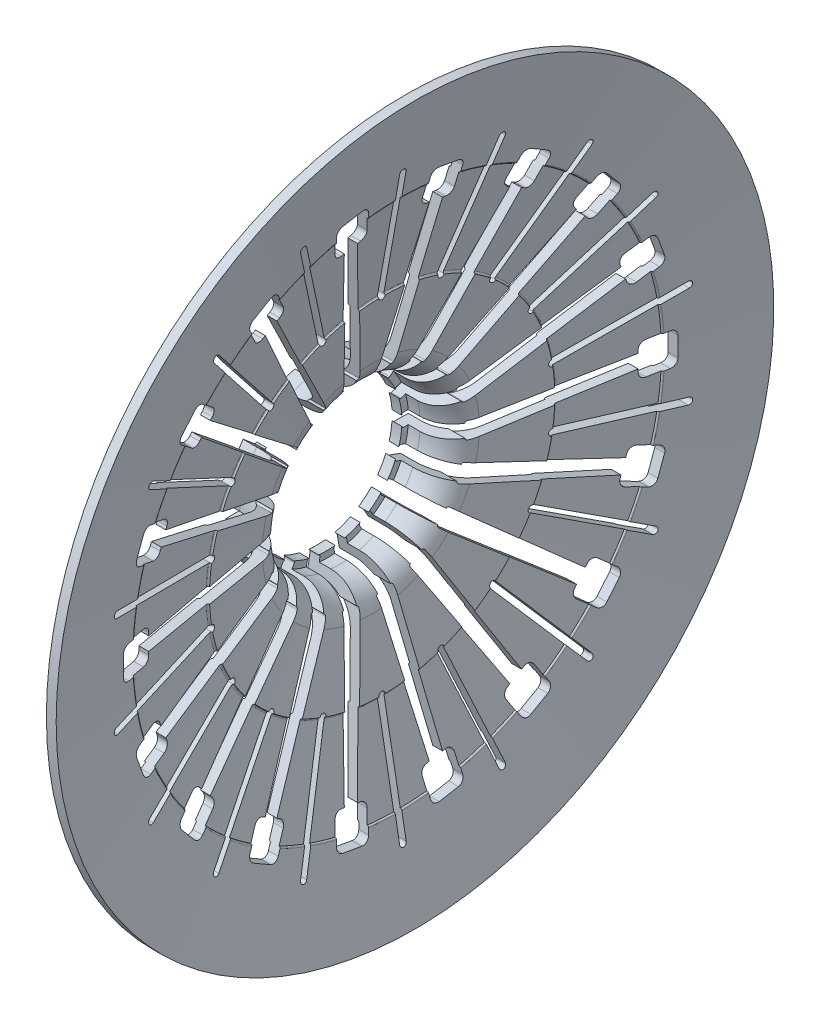
from build123d import *

# Parameters (mm, degrees)
CUT_EXTRUDE3_DEPTH = 1469.5
CUT_EXTRUDE4_DEPTH = 538.860152276
SKETCH10_R         = 23
CUT_EXTRUDE5_DEPTH = 538.860152276
CIRPATTERN3_COUNT  = 18


with BuildPart() as part:
    # Sketch2 → Revolve1 (revolve)
    with BuildSketch(Plane.XY, mode=Mode.PRIVATE) as revolve1_sk:
        with BuildLine():
            Line((1418.670249885, 525.636322255), (1415.670249885, 525.636322255))
            Line((1415.670249885, 525.636322255), (1410.645316665, 497.138509845))
            ThreePointArc((1410.645316665, 497.138509845), (1410.473894028, 496.843629316), (1410.153261537, 496.727289069))
            Line((1410.153261537, 496.727289069), (1405.181043726, 469.168980393))
            ThreePointArc((1405.181043726, 469.168980393), (1405.27005744, 468.784299802), (1405.610411969, 468.584146378))
            Line((1405.610411969, 468.584146378), (1402.668518685, 451.899840478))
            ThreePointArc((1402.668518685, 451.899840478), (1399.248317252, 445.975877824), (1392.820441155, 443.636322255))
            Line((1392.820441155, 443.636322255), (1388.670249885, 443.636322255))
            Line((1388.670249885, 443.636322255), (1388.670249885, 415.636322255))
            Line((1388.670249885, 415.636322255), (1391.670249885, 415.636322255))
            Line((1391.670249885, 415.636322255), (1391.670249885, 440.636322255))
            Line((1391.670249885, 440.636322255), (1395.291460213, 440.636322255))
            ThreePointArc((1395.291460213, 440.636322255), (1401.719336309, 442.975877824), (1405.139537743, 448.899840478))
            Line((1405.139537743, 448.899840478), (1408.610411969, 468.584146378))
            ThreePointArc((1408.610411969, 468.584146378), (1408.27005744, 468.784299802), (1408.181043726, 469.168980393))
            Line((1408.181043726, 469.168980393), (1413.153261537, 496.727289069))
            ThreePointArc((1413.153261537, 496.727289069), (1413.473894028, 496.843629316), (1413.645316665, 497.138509845))
            Line((1413.645316665, 497.138509845), (1418.670249885, 525.636322255))
        make_face()
    revolve(revolve1_sk.sketch.rotate(Axis((1325.04174439, 415.636322255, 0), (1, 0, 0)), 90), axis=Axis((1325.04174439, 415.636322255, 0), (1, 0, 0)))

    # Sketch8 → Cut-Extrude3 (cut)
    with BuildSketch(Plane(origin=(0, 0, 0), x_dir=(0, 0, -1), z_dir=(1, 0, 0))):
        with BuildLine():
            Line((1, 504.636322255), (1, 468.636322255))
            ThreePointArc((1, 468.636322255), (0, 467.636322255), (-1, 468.636322255))
            Line((-1, 468.636322255), (-1, 504.636322255))
            ThreePointArc((-1, 504.636322255), (0, 505.636322255), (1, 504.636322255))
        make_face()
        with BuildLine():
            Line((31.379485377, 498.926945361), (19.066760217, 465.098011013))
            ThreePointArc((19.066760217, 465.098011013), (17.785047453, 464.500338536), (17.187374975, 465.7820513))
            Line((17.187374975, 465.7820513), (29.500100135, 499.610985648))
            ThreePointArc((29.500100135, 499.610985648), (30.781812899, 500.208658125), (31.379485377, 498.926945361))
        make_face()
        with BuildLine():
            Line((57.974141705, 483.171490083), (34.833787757, 455.59389013))
            ThreePointArc((34.833787757, 455.59389013), (33.424955704, 455.470633297), (33.30169887, 456.87946535))
            Line((33.30169887, 456.87946535), (56.442052819, 484.457065302))
            ThreePointArc((56.442052819, 484.457065302), (57.850884872, 484.580322135), (57.974141705, 483.171490083))
        make_face()
        with BuildLine():
            Line((77.576260937, 459.270296851), (46.399346401, 441.270296851))
            ThreePointArc((46.399346401, 441.270296851), (45.033320997, 441.636322255), (45.399346401, 443.002347659))
            Line((45.399346401, 443.002347659), (76.576260937, 461.002347659))
            ThreePointArc((76.576260937, 461.002347659), (77.942286341, 460.636322255), (77.576260937, 459.270296851))
        make_face()
        with BuildLine():
            Line((87.821538196, 430.106202314), (52.368459087, 423.854867918))
            ThreePointArc((52.368459087, 423.854867918), (51.210003157, 424.666027493), (52.021162732, 425.824483424))
            Line((52.021162732, 425.824483424), (87.47424184, 432.07581782))
            ThreePointArc((87.47424184, 432.07581782), (88.632697771, 431.264658245), (87.821538196, 430.106202314))
        make_face()
        with BuildLine():
            Line((87.47424184, 399.196826689), (52.021162732, 405.448161085))
            ThreePointArc((52.021162732, 405.448161085), (51.210003157, 406.606617016), (52.368459087, 407.417776591))
            Line((52.368459087, 407.417776591), (87.821538196, 401.166442195))
            ThreePointArc((87.821538196, 401.166442195), (88.632697771, 400.007986265), (87.47424184, 399.196826689))
        make_face()
        with BuildLine():
            Line((76.576260937, 370.270296851), (45.399346401, 388.270296851))
            ThreePointArc((45.399346401, 388.270296851), (45.033320997, 389.636322255), (46.399346401, 390.002347659))
            Line((46.399346401, 390.002347659), (77.576260937, 372.002347659))
            ThreePointArc((77.576260937, 372.002347659), (77.942286341, 370.636322255), (76.576260937, 370.270296851))
        make_face()
        with BuildLine():
            Line((56.442052819, 346.815579207), (33.30169887, 374.39317916))
            ThreePointArc((33.30169887, 374.39317916), (33.424955704, 375.802011213), (34.833787757, 375.678754379))
            Line((34.833787757, 375.678754379), (57.974141705, 348.101154427))
            ThreePointArc((57.974141705, 348.101154427), (57.850884872, 346.692322374), (56.442052819, 346.815579207))
        make_face()
        with BuildLine():
            Line((29.500100135, 331.661658861), (17.187374975, 365.49059321))
            ThreePointArc((17.187374975, 365.49059321), (17.785047453, 366.772305974), (19.066760217, 366.174633496))
            Line((19.066760217, 366.174633496), (31.379485377, 332.345699148))
            ThreePointArc((31.379485377, 332.345699148), (30.781812899, 331.063986384), (29.500100135, 331.661658861))
        make_face()
        with BuildLine():
            Line((-1, 326.636322255), (-1, 362.636322255))
            ThreePointArc((-1, 362.636322255), (0, 363.636322255), (1, 362.636322255))
            Line((1, 362.636322255), (1, 326.636322255))
            ThreePointArc((1, 326.636322255), (0, 325.636322255), (-1, 326.636322255))
        make_face()
        with BuildLine():
            Line((-31.379485377, 332.345699148), (-19.066760217, 366.174633496))
            ThreePointArc((-19.066760217, 366.174633496), (-17.785047453, 366.772305974), (-17.187374975, 365.49059321))
            Line((-17.187374975, 365.49059321), (-29.500100135, 331.661658861))
            ThreePointArc((-29.500100135, 331.661658861), (-30.781812899, 331.063986384), (-31.379485377, 332.345699148))
        make_face()
        with BuildLine():
            Line((-57.974141705, 348.101154427), (-34.833787757, 375.678754379))
            ThreePointArc((-34.833787757, 375.678754379), (-33.424955704, 375.802011213), (-33.30169887, 374.39317916))
            Line((-33.30169887, 374.39317916), (-56.442052819, 346.815579207))
            ThreePointArc((-56.442052819, 346.815579207), (-57.850884872, 346.692322374), (-57.974141705, 348.101154427))
        make_face()
        with BuildLine():
            Line((-77.576260937, 372.002347659), (-46.399346401, 390.002347659))
            ThreePointArc((-46.399346401, 390.002347659), (-45.033320997, 389.636322255), (-45.399346401, 388.270296851))
            Line((-45.399346401, 388.270296851), (-76.576260937, 370.270296851))
            ThreePointArc((-76.576260937, 370.270296851), (-77.942286341, 370.636322255), (-77.576260937, 372.002347659))
        make_face()
        with BuildLine():
            Line((-87.821538196, 401.166442195), (-52.368459087, 407.417776591))
            ThreePointArc((-52.368459087, 407.417776591), (-51.210003157, 406.606617016), (-52.021162732, 405.448161085))
            Line((-52.021162732, 405.448161085), (-87.47424184, 399.196826689))
            ThreePointArc((-87.47424184, 399.196826689), (-88.632697771, 400.007986265), (-87.821538196, 401.166442195))
        make_face()
        with BuildLine():
            Line((-87.47424184, 432.07581782), (-52.021162732, 425.824483424))
            ThreePointArc((-52.021162732, 425.824483424), (-51.210003157, 424.666027493), (-52.368459087, 423.854867918))
            Line((-52.368459087, 423.854867918), (-87.821538196, 430.106202314))
            ThreePointArc((-87.821538196, 430.106202314), (-88.632697771, 431.264658245), (-87.47424184, 432.07581782))
        make_face()
        with BuildLine():
            Line((-76.576260937, 461.002347659), (-45.399346401, 443.002347659))
            ThreePointArc((-45.399346401, 443.002347659), (-45.033320997, 441.636322255), (-46.399346401, 441.270296851))
            Line((-46.399346401, 441.270296851), (-77.576260937, 459.270296851))
            ThreePointArc((-77.576260937, 459.270296851), (-77.942286341, 460.636322255), (-76.576260937, 461.002347659))
        make_face()
        with BuildLine():
            Line((-56.442052819, 484.457065302), (-33.30169887, 456.87946535))
            ThreePointArc((-33.30169887, 456.87946535), (-33.424955704, 455.470633297), (-34.833787757, 455.59389013))
            Line((-34.833787757, 455.59389013), (-57.974141705, 483.171490083))
            ThreePointArc((-57.974141705, 483.171490083), (-57.850884872, 484.580322135), (-56.442052819, 484.457065302))
        make_face()
        with BuildLine():
            Line((-29.500100135, 499.610985648), (-17.187374975, 465.7820513))
            ThreePointArc((-17.187374975, 465.7820513), (-17.785047453, 464.500338536), (-19.066760217, 465.098011013))
            Line((-19.066760217, 465.098011013), (-31.379485377, 498.926945361))
            ThreePointArc((-31.379485377, 498.926945361), (-30.781812899, 500.208658125), (-29.500100135, 499.610985648))
        make_face()
    extrude(amount=CUT_EXTRUDE3_DEPTH, mode=Mode.SUBTRACT)

    # Sketch9 → Cut-Extrude4 (cut, through all)
    with BuildSketch(Plane.ZY.offset(-1388.670249885)):
        with BuildLine():
            Line((-7.242083509, 444.822145892), (-7.179060836, 444.83325849))
            Line((-7.179060836, 444.83325849), (-6.042026252, 438.384814925))
            ThreePointArc((-6.042026252, 438.384814925), (-5.823186108, 438.053114362), (-5.431545304, 437.98578121))
            ThreePointArc((-5.431545304, 437.98578121), (-3.993908086, 438.286900574), (-2.539982114, 438.495641817))
            ThreePointArc((-2.539982114, 438.495641817), (-2.194989435, 438.692863326), (-2.10279524, 439.079407636))
            Line((-2.10279524, 439.079407636), (-3.239829824, 445.5278512))
            Line((-3.239829824, 445.5278512), (-3.176807151, 445.538963798))
            ThreePointArc((-3.176807151, 445.538963798), (-2.854055217, 445.744579456), (-2.771227363, 446.118191763))
            Line((-2.771227363, 446.118191763), (-10.993154058, 489.867669909))
            Line((-10.993154058, 489.867669909), (-10.076110622, 490.029369409))
            ThreePointArc((-10.076110622, 490.029369409), (-8.785102889, 490.851832043), (-8.453791471, 492.346281271))
            Line((-8.453791471, 492.346281271), (-9.495680537, 498.255127789))
            ThreePointArc((-9.495680537, 498.255127789), (-10.318143171, 499.546135522), (-11.812592399, 499.877446939))
            Line((-11.812592399, 499.877446939), (-14.767015658, 499.356502406))
            Line((-14.767015658, 499.356502406), (-17.721438917, 498.835557873))
            ThreePointArc((-17.721438917, 498.835557873), (-19.01244665, 498.01309524), (-19.343758067, 496.518646012))
            Line((-19.343758067, 496.518646012), (-18.301869001, 490.609799494))
            ThreePointArc((-18.301869001, 490.609799494), (-17.479406368, 489.318791761), (-15.98495714, 488.987480343))
            Line((-15.98495714, 488.987480343), (-15.06317206, 489.150015923))
            Line((-15.06317206, 489.150015923), (-7.821311475, 445.22772568))
            ThreePointArc((-7.821311475, 445.22772568), (-7.615695816, 444.904973746), (-7.242083509, 444.822145892))
        make_face()
    cut_extrude4 = extrude(amount=-CUT_EXTRUDE4_DEPTH, mode=Mode.SUBTRACT)

    # Sketch10 → Cut-Extrude5 (cut, through all)
    with BuildSketch(Plane.ZY.offset(-1388.670249885)):
        with Locations((0, 415.636322255)):
            Circle(SKETCH10_R)
    extrude(amount=-CUT_EXTRUDE5_DEPTH, mode=Mode.SUBTRACT)

    # CirPattern3: Cut-Extrude4 ×18 about axis
    cirpattern3_axis = Axis((0, 415.636322255, 0), (1, 0, 0))
    for i in range(1, CIRPATTERN3_COUNT):
        add(cut_extrude4.rotate(cirpattern3_axis, i * 360 / CIRPATTERN3_COUNT), mode=Mode.SUBTRACT)


solid = part.part
